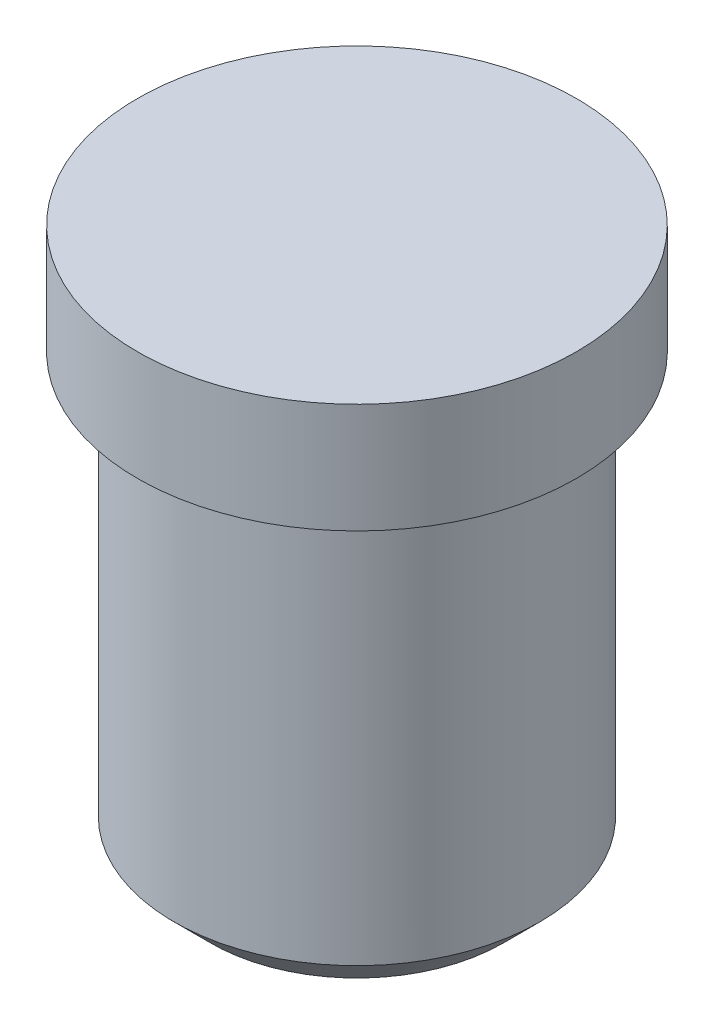
SolidWorks part; units mm, degrees
material "45"
ref_plane "Front Plane" through (0, 0, 0) normal (0, 0, 1) x (1, 0, 0)
ref_plane "Top Plane" through (0, 0, 0) normal (0, 1, 0) x (1, 0, 0)
ref_plane "Right Plane" through (0, 0, 0) normal (1, 0, 0) x (0, 0, -1)
sketch "Sketch1" plane through (0, 0, 0) normal (0, 0, 1) x (1, 0, 0)
  line L1 (104.0808, -426.8521) -> (109.0808, -426.8521)
  line L4 (109.0808, -414.8521) -> (110.0808, -414.8521)
  line L9 (104.0808, -427.3063) -> (104.0808, -411.8521) construction
  line L10 (99.0808, -422.8521) -> (99.0808, -425.1521) construction
  line L11 (109.0808, -426.8521) -> (109.0808, -414.8521)
  line L12 (116.0808, -425.1521) -> (76.3808, -425.1521) construction
  line L13 (110.0808, -414.8521) -> (110.0808, -411.8521)
  line L14 (110.0808, -411.8521) -> (104.0808, -411.8521)
  line L15 (104.0808, -411.8521) -> (104.0808, -426.8521)
  dimension "D1" = 5
  dimension "D2" = 1.7
  dimension "D3" = 10
  dimension "D4" = 12
  dimension "D5" = 3
  dimension "D6" = 12
revolve "Revolve1" add sketch "Sketch1" angle 360 about L9
chamfer "Chamfer1" distance 1 angle 45 1 edges at (109.0808, -426.8521, 0)
